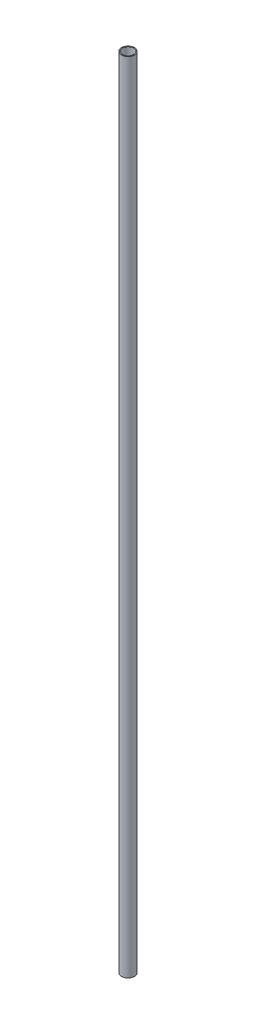
from build123d import *

# Parameters (mm, degrees)
SWEEP_THIN1_PROFILE_R   = 15
SWEEP_THIN1_PROFILE_R_2 = 13


with BuildPart() as part:
    # Sweep-Thin1: sweep along a path in Sketch1
    with BuildLine(Plane.XY) as sweep_thin1_path:
        Line((0, 0), (0, 1846.4))
    # Sweep-Thin1 profile (on start of the path) → Sweep-Thin1 (sweep)
    with BuildSketch(Plane.ZX):
        Circle(SWEEP_THIN1_PROFILE_R)
        Circle(SWEEP_THIN1_PROFILE_R_2, mode=Mode.SUBTRACT)
    sweep(path=sweep_thin1_path.line)


solid = part.part
